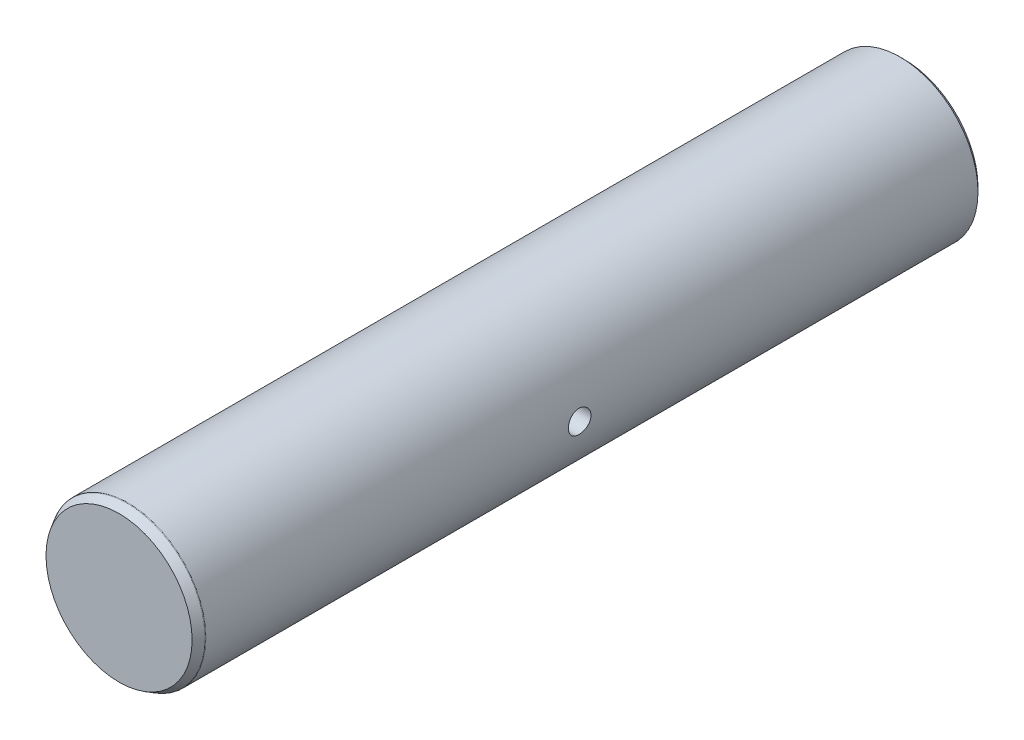
SolidWorks part; units mm, degrees
material "普通碳钢"
ref_plane "前视" through (0, 0, 0) normal (0, 0, 1) x (1, 0, 0)
ref_plane "上视" through (0, 0, 0) normal (0, 1, 0) x (1, 0, 0)
ref_plane "右视" through (0, 0, 0) normal (1, 0, 0) x (0, 0, -1)
sketch "草图1" plane through (0, 0, 0) normal (0, 0, 1) x (1, 0, 0)
  line L0 (-59.9479, 0) -> (67.7736, 0) construction
  line L1 (0, 44.9609) -> (0, -43.3367) construction
  circle A0 centre (0, 0) radius 27.5
  dimension "D1" = 55
extrude "凸台-拉伸1" add sketch "草图1" along normal blind 277
hole_wizard "大小mm 暗销孔1" positions "草图3" profile "草图2" hole size "Ø6.0" standard "GB"
sketch "草图3" plane through (0, 0, 0) normal (0, 0, 1) x (1, 0, 0)
  line L0 (50, 0) -> (-50, 0) construction
  point P0 (15, 0)
  point P2 (-15, 0)
  dimension "D1" = 15
  dimension "D2" = 15
sketch "草图2" plane through (15, 0, 0) normal (1, 0, 0) x (0, 1, 0)
  line L0 (0, 0) -> (0, 11.8026)
  line L1 (0, 11.8026) -> (3, 10)
  line L2 (3, 10) -> (3, 0)
  line L5 (3, 0) -> (0, 0)
  line L10 (0, 11.8026) -> (-3, 10) construction
  line L11 (0, -6.35) -> (0, 107.95) construction
  dimension "孔直径" = 6
  dimension "孔深度" = 10
  dimension "导头角度" = 118
ref_plane "基准面1" through (27.5, 0, 0) normal (1, 0, 0) x (0, 0, -1)
hole_wizard "大小mm 暗销孔2" positions "草图5" profile "草图4" hole size "Ø8.0" standard "GB"
sketch "草图5" plane through (27.5, 0, 0) normal (1, 0, 0) x (0, 0, -1)
  line L1 (50, 0) -> (-50, 0) construction
  line L2 (0, 50) -> (0, -50) construction
  point P0 (-142, 0)
  dimension "D1" = 142
sketch "草图4" plane through (27.5, 0, 142) normal (0, 1, 0) x (0, 0, -1)
  line L0 (0, 0) -> (0, 10.4034)
  line L1 (0, 10.4034) -> (4, 8)
  line L2 (4, 8) -> (4, 0)
  line L5 (4, 0) -> (0, 0)
  line L10 (0, 10.4034) -> (-4, 8) construction
  line L11 (0, -6.35) -> (0, 107.95) construction
  dimension "孔直径" = 8
  dimension "孔深度" = 8
  dimension "导头角度" = 118
chamfer "倒角1" distance 1.5 angle 45 1 edges at (27.5, 0, 0)
chamfer "倒角2" distance 3 angle 30 1 edges at (27.5, 0, 277)
fillet "圆角1" radius 0.5 1 edges at (27.5, 0, 274)
